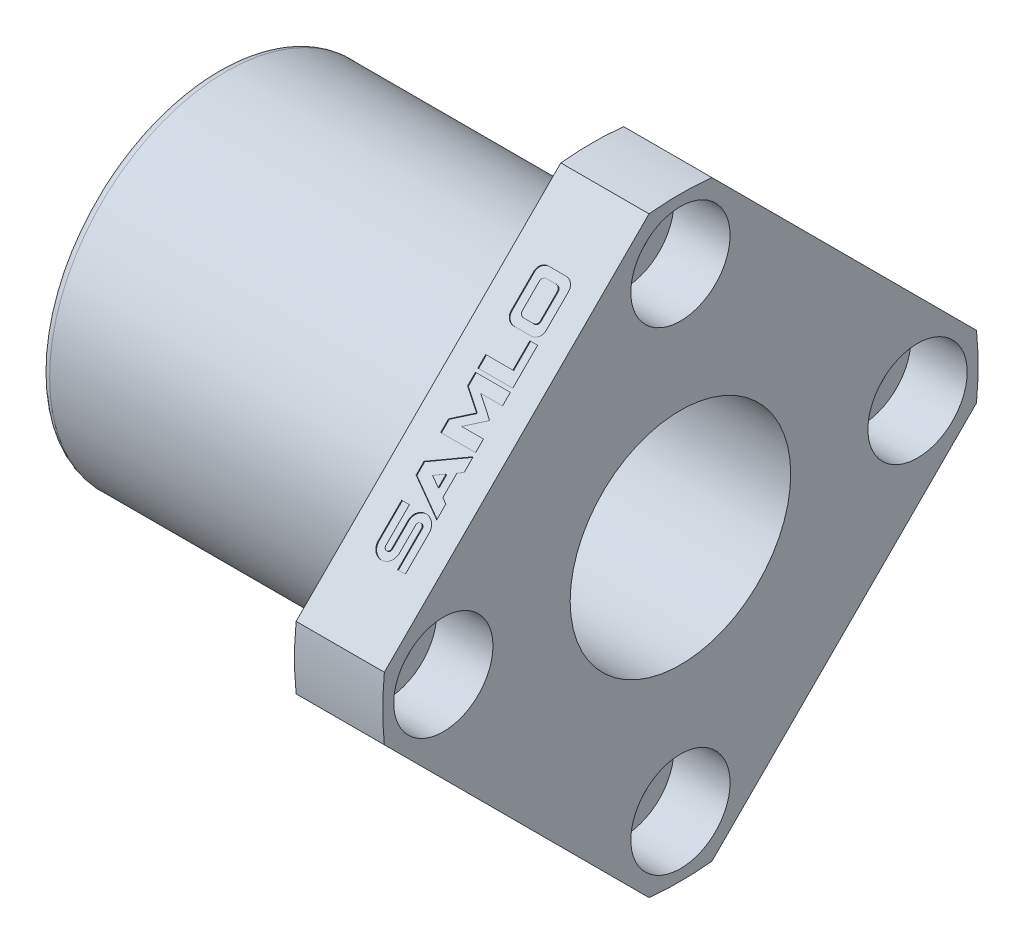
from build123d import *

# Parameters (mm, degrees)
SKETCH2_R            = 27
SKETCH2_R_2          = 2.75
SKETCH2_R_3          = 10
BOSS_EXTRUDE1_DEPTH  = 8
SKETCH3_R            = 4.5
CUT_EXTRUDE1_DEPTH   = 5.1
LPATTERN1_COUNT      = 2
LPATTERN1_PITCH      = 30.405591591
LPATTERN1_COUNT_DIR2 = 2
LPATTERN1_PITCH_DIR2 = 30.405591591
SKETCH5_R            = 54
CUT_EXTRUDE2_DEPTH   = 8
CUT_EXTRUDE3_DEPTH   = 0.1
CUT_EXTRUDE4_DEPTH   = 0.1
CUT_EXTRUDE5_DEPTH   = 0.1
CUT_EXTRUDE6_DEPTH   = 0.1
CUT_EXTRUDE7_DEPTH   = 0.1


with BuildPart() as part:
    # Sketch1 → Revolve1 (revolve)
    with BuildSketch(Plane.XY, mode=Mode.PRIVATE) as revolve1_sk:
        with BuildLine():
            Line((0, 10), (42, 10))
            Line((42, 10), (42, 15.2))
            ThreePointArc((42, 15.2), (41.765685425, 15.765685425), (41.2, 16))
            Line((41.2, 16), (0.8, 16))
            ThreePointArc((0.8, 16), (0.234314575, 15.765685425), (0, 15.2))
            Line((0, 15.2), (0, 10))
        make_face()
    revolve(revolve1_sk.sketch.rotate(Axis((42, 0, 0), (-1, 0, 0)), 270), axis=Axis((42, 0, 0), (-1, 0, 0)))

    # Sketch2 → Boss-Extrude1 (add)
    with BuildSketch(Plane(origin=(42, 0, 0), x_dir=(0, 0, -1), z_dir=(1, 0, 0))):
        Circle(SKETCH2_R)
        with Locations((21.5, 0)):
            Circle(SKETCH2_R_2, mode=Mode.SUBTRACT)
        with Locations((0, 21.5)):
            Circle(SKETCH2_R_2, mode=Mode.SUBTRACT)
        with Locations((0, -21.5)):
            Circle(SKETCH2_R_2, mode=Mode.SUBTRACT)
        with Locations(Location((0, 0, 0), (0, 0, 180))):
            Circle(SKETCH2_R_3, mode=Mode.SUBTRACT)
        with Locations((-21.5, 0)):
            Circle(SKETCH2_R_2, mode=Mode.SUBTRACT)
    extrude(amount=-BOSS_EXTRUDE1_DEPTH)

    # Sketch3 → Cut-Extrude1 (cut)
    with BuildSketch(Plane(origin=(42, 0, 0), x_dir=(0, 0, -1), z_dir=(1, 0, 0))):
        with Locations((0, 21.5)):
            Circle(SKETCH3_R)
    cut_extrude1 = extrude(amount=-CUT_EXTRUDE1_DEPTH, mode=Mode.SUBTRACT)

    # LPattern1: Cut-Extrude1 2 × 2
    with Locations(*[Vector(0, -0.7071067811865475, 0.7071067811865477) * (i * LPATTERN1_PITCH) + Vector(0, -0.7071067811865477, -0.7071067811865474) * (j * LPATTERN1_PITCH_DIR2) for i in range(LPATTERN1_COUNT) for j in range(LPATTERN1_COUNT_DIR2) if (i, j) != (0, 0)]):
        add(cut_extrude1, mode=Mode.SUBTRACT)

    # Sketch5 → Cut-Extrude2 (cut)
    with BuildSketch(Plane(origin=(42, 0, 0), x_dir=(0, 0, -1), z_dir=(1, 0, 0))):
        Circle(SKETCH5_R)
        Polygon((-29.69848481, 0), (0, -29.69848481), (29.69848481, 0), (0, 29.69848481), align=None, mode=Mode.SUBTRACT)
    extrude(amount=-CUT_EXTRUDE2_DEPTH, mode=Mode.SUBTRACT)

    # Sketch6 → Cut-Extrude3 (cut)
    with BuildSketch(Plane(origin=(0, 14.849242405, 14.849242405), x_dir=(1, 0, 0), z_dir=(0, 0.7071067811865477, 0.7071067811865475))):
        with BuildLine():
            Line((38.352971429, -9.883885714), (38.352971429, -7.780571429))
            ThreePointArc((38.352971429, -7.780571429), (38.6164, -7.517142857), (38.879828571, -7.780571429))
            Line((38.879828571, -7.780571429), (38.879828571, -10.8496))
            Line((38.879828571, -10.8496), (39.582, -10.8496))
            Line((39.582, -10.8496), (39.582, -7.780571429))
            ThreePointArc((39.582, -7.780571429), (38.6164, -6.829713846), (37.6508, -7.780571429))
            Line((37.6508, -7.780571429), (37.6508, -9.883885714))
            ThreePointArc((37.6508, -9.883885714), (37.387371429, -10.147314286), (37.123942857, -9.883885714))
            Line((37.123942857, -9.883885714), (37.123942857, -6.860114286))
            Line((37.123942857, -6.860114286), (36.421771429, -6.860114286))
            Line((36.421771429, -6.860114286), (36.421771429, -9.883885714))
            ThreePointArc((36.421771429, -9.883885714), (37.387371429, -10.834743297), (38.352971429, -9.883885714))
        make_face()
    extrude(amount=-CUT_EXTRUDE3_DEPTH, mode=Mode.SUBTRACT)

    # Sketch7 → Cut-Extrude4 (cut)
    with BuildSketch(Plane(origin=(0, 14.849242405, 14.849242405), x_dir=(1, 0, 0), z_dir=(0, 0.7071067811865477, 0.7071067811865475))):
        Polygon((36.414228571, -5.000457143), (39.5804, -6.828342857), (39.5804, -5.664914286), (39.118914286, -5.398628571), (39.118914286, -3.588342857), (39.5804, -3.321828571), (39.5804, -2.158628571), (36.414228571, -3.986285714), align=None)
        Polygon((37.551142857, -4.493485714), (38.416742857, -4.993142857), (38.416742857, -3.9936), align=None, mode=Mode.SUBTRACT)
    extrude(amount=-CUT_EXTRUDE4_DEPTH, mode=Mode.SUBTRACT)

    # Sketch8 → Cut-Extrude5 (cut)
    with BuildSketch(Plane(origin=(0, 14.849242405, 14.849242405), x_dir=(1, 0, 0), z_dir=(0, 0.7071067811865477, 0.7071067811865475))):
        Polygon((36.416057143, 2.612114286), (36.416057143, 1.604571429), (38.089428571, 0.381485714), (36.416057143, -0.841828571), (36.416057143, -1.849371429), (39.582, -1.849371429), (39.582, -0.841828571), (37.606, -0.841828571), (39.279371429, 0.381485714), (37.606, 1.604571429), (39.5804, 1.604571429), (39.5804, 2.612114286), align=None)
    extrude(amount=-CUT_EXTRUDE5_DEPTH, mode=Mode.SUBTRACT)

    # Sketch9 → Cut-Extrude6 (cut)
    with BuildSketch(Plane(origin=(0, 14.849242405, 14.849242405), x_dir=(1, 0, 0), z_dir=(0, 0.7071067811865477, 0.7071067811865475))):
        Polygon((36.416057143, 2.917485714), (39.582, 2.917485714), (39.582, 6.101485714), (38.879828571, 6.101485714), (38.879828571, 3.925028571), (36.416057143, 3.925028571), align=None)
    extrude(amount=-CUT_EXTRUDE6_DEPTH, mode=Mode.SUBTRACT)

    # Sketch10 → Cut-Extrude7 (cut)
    with BuildSketch(Plane(origin=(0, 14.849242405, 14.849242405), x_dir=(1, 0, 0), z_dir=(0, 0.7071067811865477, 0.7071067811865475))):
        with BuildLine():
            Line((36.421771429, 10.072685714), (36.421771429, 7.183542857))
            ThreePointArc((36.421771429, 7.183542857), (36.649923534, 6.635009248), (37.198457143, 6.406857143))
            Line((37.198457143, 6.406857143), (38.805314286, 6.406857143))
            ThreePointArc((38.805314286, 6.406857143), (39.353847895, 6.635009248), (39.582, 7.183542857))
            Line((39.582, 7.183542857), (39.582, 10.072685714))
            ThreePointArc((39.582, 10.072685714), (39.353928291, 10.621366852), (38.805314286, 10.8496))
            Line((38.805314286, 10.8496), (37.198457143, 10.8496))
            ThreePointArc((37.198457143, 10.8496), (36.649843138, 10.621366852), (36.421771429, 10.072685714))
        make_face()
        with BuildLine():
            Line((37.552971429, 7.170057143), (38.450571429, 7.170057143))
            ThreePointArc((38.450571429, 7.170057143), (38.709322389, 7.277706182), (38.816971429, 7.536457143))
            Line((38.816971429, 7.536457143), (38.816971429, 9.719771429))
            ThreePointArc((38.816971429, 9.719771429), (38.709322389, 9.978522389), (38.450571429, 10.086171429))
            Line((38.450571429, 10.086171429), (37.552971429, 10.086171429))
            ThreePointArc((37.552971429, 10.086171429), (37.294367965, 9.978442068), (37.1868, 9.719771429))
            Line((37.1868, 9.719771429), (37.1868, 7.536457143))
            ThreePointArc((37.1868, 7.536457143), (37.294367965, 7.277786503), (37.552971429, 7.170057143))
        make_face(mode=Mode.SUBTRACT)
    extrude(amount=-CUT_EXTRUDE7_DEPTH, mode=Mode.SUBTRACT)


solid = part.part
